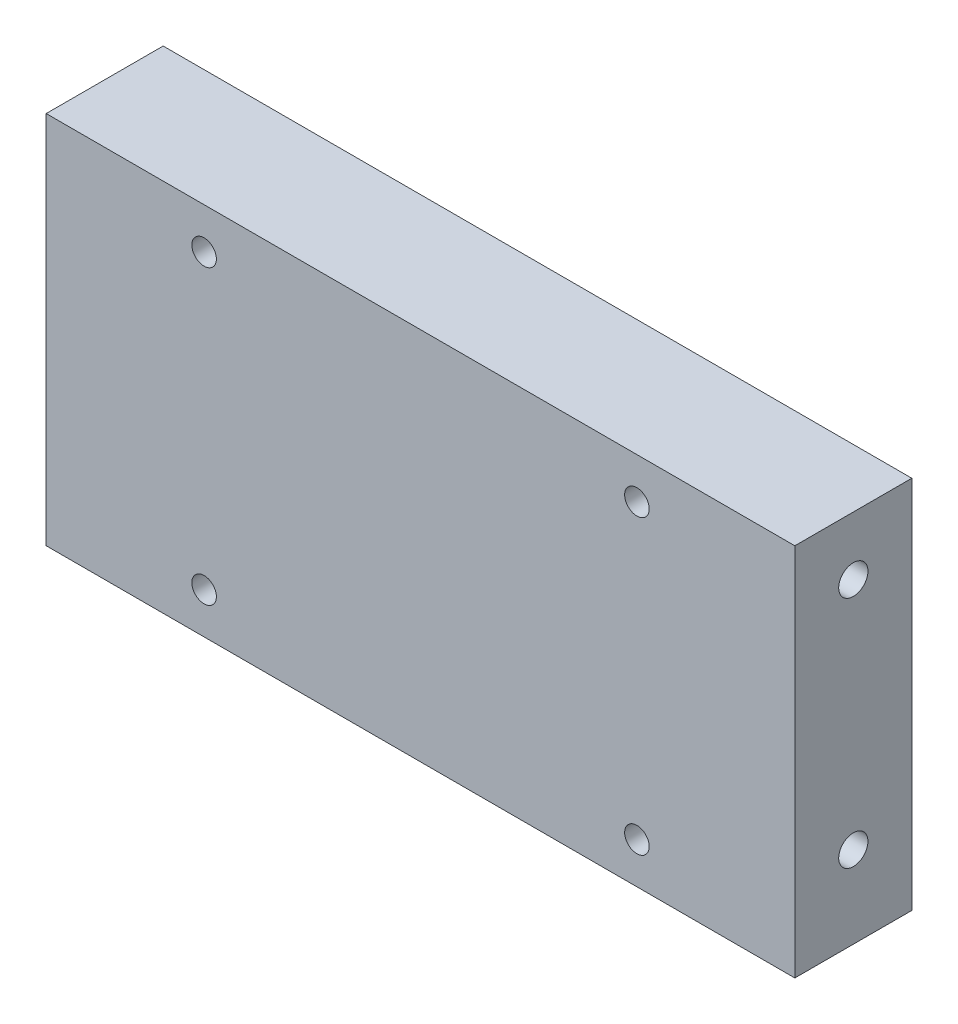
from build123d import *

# Parameters (mm, degrees)
SKETCH_1_W             = 128
SKETCH_1_H             = 64
EXTRUDE_1_DEPTH        = 20
HOLE_WIZARD_M5_1_D     = 4.2
PATTERN_LINEAR_1_COUNT = 2
PATTERN_LINEAR_1_PITCH = 40


with BuildPart() as part:
    # 草图1 → 拉伸1 (new body)
    with BuildSketch(Plane.XY):
        with Locations((64, 32)):
            Rectangle(SKETCH_1_W, SKETCH_1_H)
    extrude(amount=EXTRUDE_1_DEPTH)

    # M5 螺纹孔1 (through all)
    with Locations(Plane.XY.offset(20)):
        with Locations((27, 57), (27, 7), (101, 7), (101, 57)):
            Hole(HOLE_WIZARD_M5_1_D / 2)

    # 草图4 → M5x0.8 螺纹孔1 (revolve, cut)
    with BuildSketch(Plane(origin=(0, 54, 10), x_dir=(0, 0, 1), z_dir=(0, 1, 0))):
        Polygon((0, 0), (0, 18.6618073), (2.1, 17.4), (2.1, 15), (2.5, 15), (2.5, 0), align=None)
    m5x0_8_1 = revolve(axis=Axis((-6.35, 54, 10), (1, 0, 0)), mode=Mode.SUBTRACT)

    # 镜向1: M5x0.8 螺纹孔1 across plane
    add(m5x0_8_1.mirror(Plane(origin=(64, 0, 0), x_dir=(0, 0, 1), z_dir=(1, 0, 0))), mode=Mode.SUBTRACT)

    # 阵列(线性)1: M5x0.8 螺纹孔1 ×2
    with Locations(*[(0, -i * PATTERN_LINEAR_1_PITCH, 0) for i in range(1, PATTERN_LINEAR_1_COUNT)]):
        add(m5x0_8_1, mode=Mode.SUBTRACT)

    # 镜向2 copy 1 sketch → 镜向2 copy 1 (revolve, cut)
    with BuildSketch(Plane(origin=(128, 14, 10), x_dir=(0, 0, 1), z_dir=(0, 1, 0))):
        Polygon((0, 0), (0, -18.6618073), (2.1, -17.4), (2.1, -15), (2.5, -15), (2.5, 0), align=None)
    revolve(axis=Axis((134.35, 14, 10), (1, 0, 0)), mode=Mode.SUBTRACT)

    # 镜向2 copy 2 sketch → 镜向2 copy 2 (revolve, cut)
    with BuildSketch(Plane(origin=(128, 54, 10), x_dir=(0, 0, 1), z_dir=(0, 1, 0))):
        Polygon((0, 0), (0, -18.6618073), (2.1, -17.4), (2.1, -15), (2.5, -15), (2.5, 0), align=None)
    revolve(axis=Axis((134.35, 54, 10), (1, 0, 0)), mode=Mode.SUBTRACT)


solid = part.part
